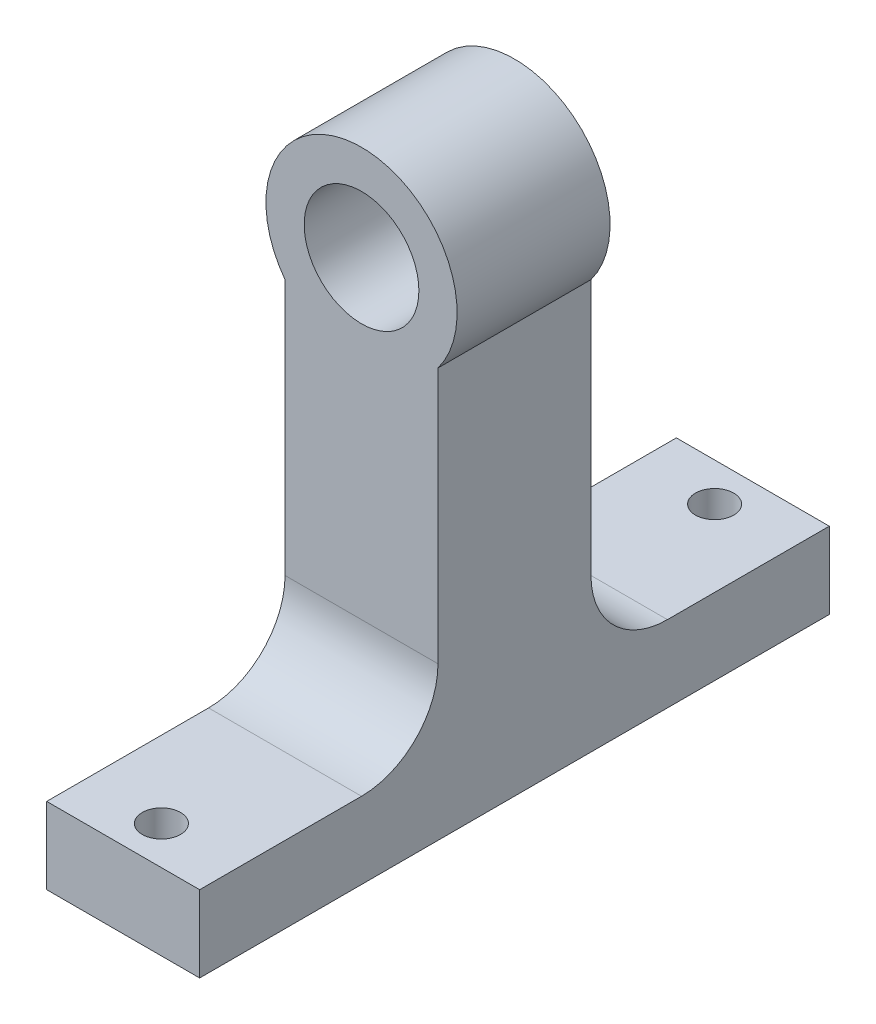
from build123d import *

# Parameters (mm, degrees)
SKETCH_1_R           = 12.5
SKETCH_1_R_2         = 7.5
EXTRUDE_1_DEPTH      = 10
EXTRUDE_3_DEPTH      = 10
EXTRUDE_4_REACH      = 66.833
EXTRUDE_4_END_RADIUS = 12.5
SKETCH_6_W           = 20
SKETCH_6_H           = 20
HOLE_WIZARD_M6_1_D   = 5


with BuildPart() as part:
    # 草图1 → 凸台-拉伸1 (new, symmetric)
    with BuildSketch(Plane.XY):
        Circle(SKETCH_1_R)
        Circle(SKETCH_1_R_2, mode=Mode.SUBTRACT)
    extrude(amount=EXTRUDE_1_DEPTH, both=True)



with BuildPart() as body_2:
    # 草图5 → 凸台-拉伸3 (new, symmetric)
    with BuildSketch(Plane(origin=(0, 0, 0), x_dir=(0, 0, -1), z_dir=(1, 0, 0))):
        with BuildLine():
            Line((21.657691454, -51), (41.168402769, -51))
            Line((41.168402769, -51), (41.168402769, -61))
            Line((41.168402769, -61), (-41.168402769, -61))
            Line((-41.168402769, -61), (-41.168402769, -51))
            Line((-41.168402769, -51), (-21.657691454, -51))
            Line((-21.657691454, -51), (-20, -51))
            ThreePointArc((-20, -51), (-12.928932188, -48.071067812), (-10, -41))
            Line((-10, -41), (-10, -12.5))
            Line((-10, -12.5), (10, -12.5))
            Line((10, -12.5), (10, -41))
            ThreePointArc((10, -41), (12.928932188, -48.071067812), (20, -51))
            Line((20, -51), (21.657691454, -51))
        make_face()
    extrude(amount=EXTRUDE_3_DEPTH, both=True)


with BuildPart() as part_1:
    add(part.part)

    add(body_2.part)  # 凸台-拉伸4 merges body 2
    # 凸台-拉伸4: up to this cylinder (the profile starts outside it)
    extrude_4_end = Plane(origin=(0, 0, 0), z_dir=(0, 0, -1)) * Cylinder(EXTRUDE_4_END_RADIUS, 159.666, mode=Mode.PRIVATE)
    # 草图6 → 凸台-拉伸4 (add, up to the surface)
    with BuildSketch(Plane(origin=(0, -12.5, 0), x_dir=(1, 0, 0), z_dir=(0, 1, 0)), mode=Mode.PRIVATE) as extrude_4_sk1:
        Rectangle(SKETCH_6_W, SKETCH_6_H)
    extrude_4_tool1 = extrude(extrude_4_sk1.sketch, amount=EXTRUDE_4_REACH, mode=Mode.PRIVATE) - extrude_4_end
    add(extrude_4_tool1.solids().sort_by_distance((0, -12.5, 0))[0])
    add(extrude_4_tool1.solids().sort_by_distance((0, -12.5, 0))[1])

    # M6 螺纹孔1 (through all)
    with Locations(Plane(origin=(0, -51, 36.168402769), x_dir=(0, 0, 1), z_dir=(0, 1, 0))):
        with Locations((0, 0)):
            hole_wizard_m6_1 = Hole(HOLE_WIZARD_M6_1_D / 2)

    # 镜向1: M6 螺纹孔1 across plane
    add(hole_wizard_m6_1.mirror(Plane.XY), mode=Mode.SUBTRACT)


solid = part_1.part
